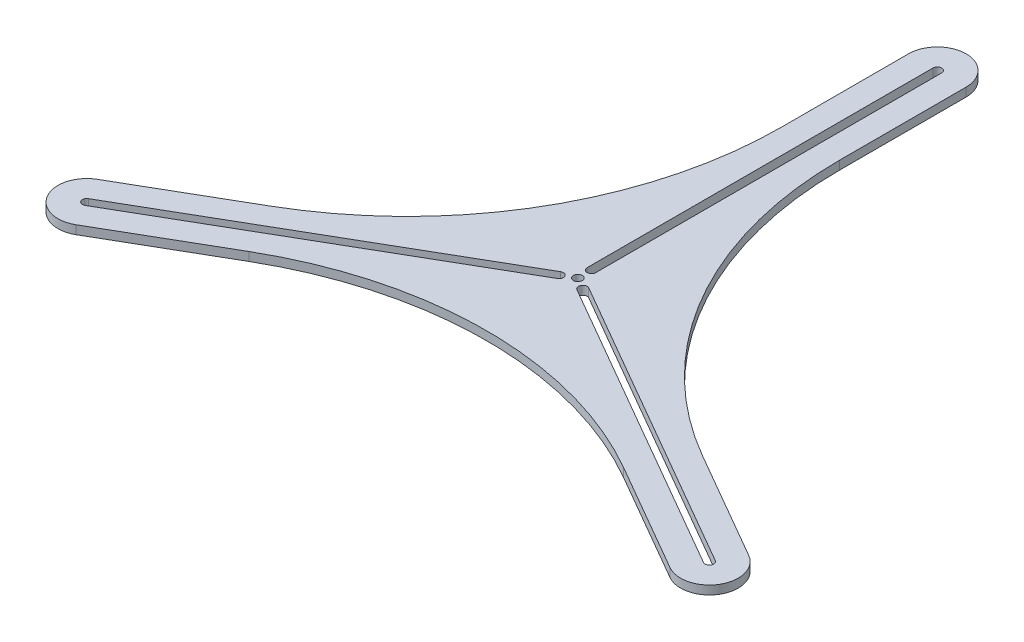
SolidWorks part; units mm, degrees
ref_plane "Front Plane" through (0, 0, 0) normal (0, 0, 1) x (1, 0, 0)
ref_plane "Top Plane" through (0, 0, 0) normal (0, 1, 0) x (1, 0, 0)
ref_plane "Right Plane" through (0, 0, 0) normal (1, 0, 0) x (0, 0, -1)
sketch "Sketch1" plane through (0, 0, 0) normal (0, 1, 0) x (1, 0, 0)
  line L0 (0, 0) -> (12.5574, 21.75) construction
  line L1 (12.5574, 21.75) -> (25.1147, 0) construction
  line L2 (25.1147, 0) -> (0, 0) construction
  line L3 (12.5574, 21.75) -> (12.5574, -50.6759) construction
  line L4 (-7.4426, 168.9081) -> (-7.4426, 256.75)
  line L5 (32.5574, 168.9081) -> (32.5574, 256.75)
  line L6 (162.5574, -56.2585) -> (238.6307, -100.1795)
  line L7 (-137.4426, -56.2585) -> (-213.516, -100.1795)
  line L8 (142.5574, -90.8995) -> (218.6307, -134.8205)
  line L9 (-117.4426, -90.8995) -> (-193.516, -134.8205)
  line L10 (4.3301, 2.5) -> (-203.516, -117.5) construction
  line L11 (4.3301, 2.5) -> (-203.516, -117.5) construction
  line L12 (5.8301, -0.0981) -> (-202.016, -120.0981)
  line L13 (2.8301, 5.0981) -> (-205.016, -114.9019)
  line L14 (-213.516, -100.1795) -> (-193.516, -134.8205) construction
  line L15 (20.7846, 2.5) -> (228.6307, -117.5) construction
  line L16 (22.2846, 5.0981) -> (230.1307, -114.9019)
  line L17 (19.2846, -0.0981) -> (227.1307, -120.0981)
  line L18 (12.5574, 16.75) -> (12.5574, 256.75) construction
  line L19 (9.5574, 16.75) -> (9.5574, 256.75)
  line L20 (15.5574, 16.75) -> (15.5574, 256.75)
  line L21 (25.1147, 0) -> (-28.4071, 30.9009) construction
  line L22 (4.3301, 2.5) -> (58.4726, 33.7592) construction
  circle A0 centre (12.5574, 16.75) radius 2.5 construction
  circle A1 centre (4.3301, 2.5) radius 2.5 construction
  circle A2 centre (20.7846, 2.5) radius 2.5 construction
  circle A3 centre (12.5574, 7.25) radius 12 construction
  circle A4 centre (12.5574, 7.25) radius 3.1
  arc A5 (5.8301, -0.0981) -> (2.8301, 5.0981) centre (4.3301, 2.5) ccw
  arc A6 (-205.016, -114.9019) -> (-202.016, -120.0981) centre (-203.516, -117.5) ccw
  arc A7 (-213.516, -100.1795) -> (-193.516, -134.8205) centre (-203.516, -117.5) ccw
  arc A8 (22.2846, 5.0981) -> (19.2846, -0.0981) centre (20.7846, 2.5) ccw
  arc A9 (227.1307, -120.0981) -> (230.1307, -114.9019) centre (228.6307, -117.5) ccw
  arc A10 (9.5574, 16.75) -> (15.5574, 16.75) centre (12.5574, 16.75) ccw
  arc A11 (15.5574, 256.75) -> (9.5574, 256.75) centre (12.5574, 256.75) ccw
  arc A12 (238.6307, -100.1795) -> (218.6307, -134.8205) centre (228.6307, -117.5) cw
  arc A13 (-7.4426, 256.75) -> (32.5574, 256.75) centre (12.5574, 256.75) cw
  arc A14 (-117.4426, -90.8995) -> (142.5574, -90.8995) centre (12.5574, -316.0662) cw
  arc A15 (162.5574, -56.2585) -> (32.5574, 168.9081) centre (292.5574, 168.9081) cw
  arc A16 (-7.4426, 168.9081) -> (-137.4426, -56.2585) centre (-267.4426, 168.9081) cw
  point P23 (-99.5929, -57.5)
  point P31 (124.7077, -57.5)
  point P38 (12.5574, 136.75)
  point P49 (12.5574, -15.844)
  point P52 (32.5574, 18.797)
  point P55 (-7.4426, 18.797)
  dimension "D3" = 5
  dimension "D4" = 24
  dimension "D5" = 6.2
  dimension "D13" = 260
  dimension "D1" = 60
  dimension "D2" = 60
  dimension "D6" = 120
  dimension "D7" = 120
  dimension "D8" = 240
  dimension "D9" = 6
  dimension "D10" = 40
  dimension "D11" = 40
  dimension "D12" = 40
extrude "Boss-Extrude2" add sketch "Sketch1" along normal blind 6
